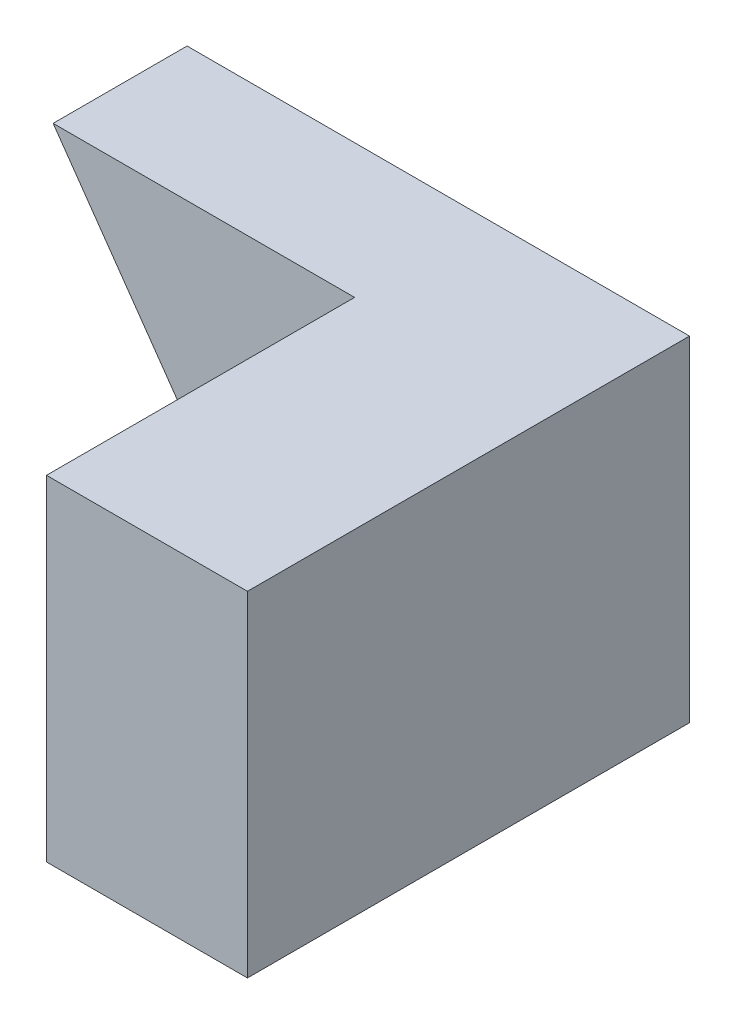
SolidWorks part; units mm, degrees
ref_plane "Front Plane" through (0, 0, 0) normal (0, 0, 1) x (1, 0, 0)
ref_plane "Top Plane" through (0, 0, 0) normal (0, 1, 0) x (1, 0, 0)
ref_plane "Right Plane" through (0, 0, 0) normal (1, 0, 0) x (0, 0, -1)
other "Configuration Table"
sketch "Sketch1" plane through (0, 0, 0) normal (0, 0, 1) x (1, 0, 0)
  line L0 (0, 0) -> (-1.7505, 2.5)
  line L1 (-1.7505, 2.5) -> (2, 2.5)
  line L2 (2, 2.5) -> (2, 0)
  line L3 (2, 0) -> (0, 0)
  dimension "D1" = 2.5
  dimension "D2" = 35
  dimension "D3" = 2
extrude "Boss-Extrude1" add sketch "Sketch1" along normal blind 1
sketch "Sketch2" plane through (0, 0, 1) normal (0, 0, 1) x (1, 0, 0)
  line L0 (2, 2.5) -> (-1.7505, 2.5) construction
  line L1 (2, 2.5) -> (0.5, 2.5)
  line L2 (2, 2.5) -> (2, 0)
  line L3 (2, 0) -> (0.5, 0)
  line L4 (0.5, 2.5) -> (0.5, 0)
  dimension "D1" = 1.5
extrude "Boss-Extrude2" add sketch "Sketch2" along normal blind 2.3
